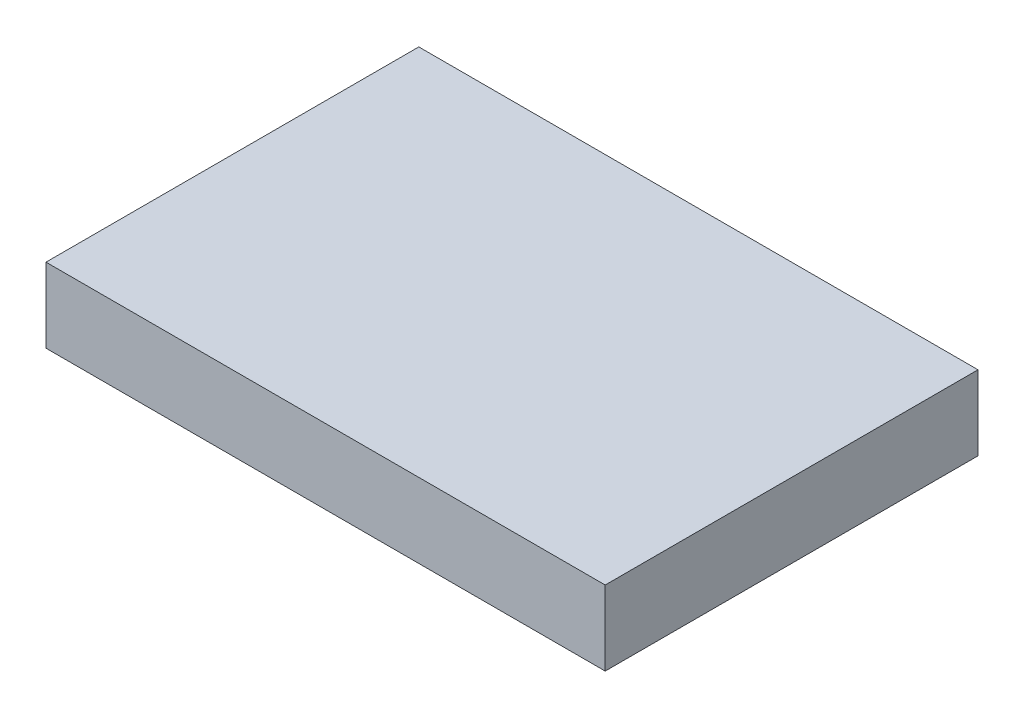
from build123d import *

# Parameters (mm, degrees)
SKETCH_1_W      = 75
SKETCH_1_H      = 50
EXTRUDE_1_DEPTH = 10


with BuildPart() as part:
    # 草图1 → 凸台-拉伸1 (new body)
    with BuildSketch(Plane(origin=(0, 0, 0), x_dir=(1, 0, 0), z_dir=(0, 1, 0))):
        Rectangle(SKETCH_1_W, SKETCH_1_H)
    extrude(amount=EXTRUDE_1_DEPTH)


solid = part.part
